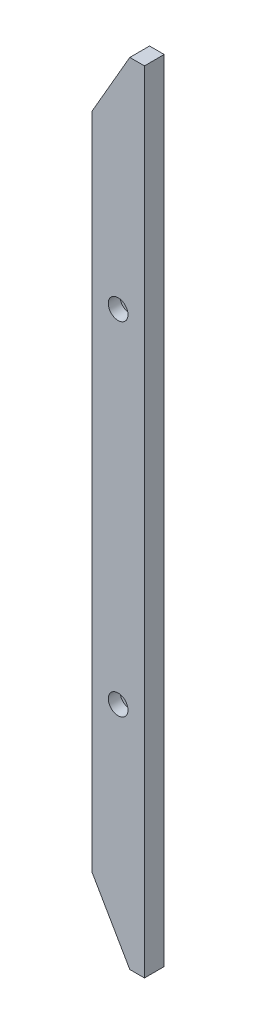
SolidWorks part; units mm, degrees
ref_plane "前视基准面" through (0, 0, 0) normal (0, 0, 1) x (1, 0, 0)
ref_plane "上视基准面" through (0, 0, 0) normal (0, 1, 0) x (1, 0, 0)
ref_plane "右视基准面" through (0, 0, 0) normal (1, 0, 0) x (0, 0, -1)
sketch "草图1" plane through (0, 0, 0) normal (0, 0, 1) x (1, 0, 0)
  line L1 (20, -300) -> (-20, -300)
  line L2 (20, -300) -> (20, 300)
  line L3 (20, 300) -> (-20, 300)
  line L4 (-20, -300) -> (-20, 300)
  line L5 (20, -300) -> (-20, 300) construction
  line L6 (20, 300) -> (-20, -300) construction
  point P0 (0, 0)
  dimension "D1" = 40
  dimension "D2" = 600
extrude "凸台-拉伸1" add sketch "草图1" along normal blind 15
hole_wizard "打孔尺寸(%根据)内六角圆柱头螺钉的类型1" positions "草图2" profile "草图3" counterbore size "M8" standard "GB" end condition up to next
sketch "草图2" plane through (0, 0, 15) normal (0, 0, 1) x (1, 0, 0)
  line L0 (0, -130) -> (0, 0) construction
  line L1 (0, 0) -> (0, 130) construction
  point P0 (0, -130)
  point P2 (0, 130)
  dimension "D1" = 130
sketch "草图3" plane through (0, -130, 15) normal (1, 0, 0) x (0, -1, 0)
  line L0 (0, 0) -> (0, 15)
  line L1 (0, 15) -> (4.5, 15)
  line L3 (4.5, 15) -> (4.5, 9)
  line L4 (4.5, 9) -> (7.5, 9)
  line L5 (7.5, 9) -> (7.5, 0)
  line L7 (7.5, 0) -> (0, 0)
  line L11 (0, -6.35) -> (0, 107.95) construction
  dimension "通孔孔直径" = 9
  dimension "通孔孔深度" = 15
  dimension "柱形沉头孔直径" = 15
  dimension "柱形沉头孔深度" = 9
chamfer "倒角1" distance 50 angle 30 2 edges at (-20, 300, 7.5) (-20, -300, 7.5)
